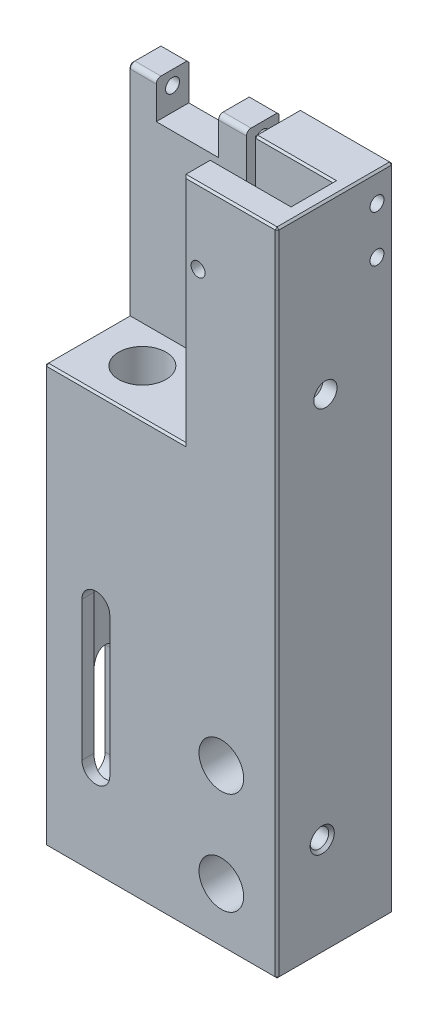
from build123d import *

# Parameters (mm, degrees)
SKETCH1_W                                         = 25
SKETCH1_H                                         = 70
BOSS_EXTRUDE1_DEPTH                               = 6.25
SKETCH2_R                                         = 4
CUT_EXTRUDE1_DEPTH                                = 35
SKETCH3_R                                         = 2.55
CUT_EXTRUDE2_DEPTH                                = 38.687033579
SKETCH5_W                                         = 9
SKETCH5_H                                         = 25
CUT_EXTRUDE3_DEPTH                                = 15
CUT_EXTRUDE4_DEPTH                                = 5
SKETCH7_R                                         = 1.75
CUT_EXTRUDE5_DEPTH                                = 6
HOLE_SIZE_PER_HEX_SOCKET_SCREW_TYPE_1_D           = 4.8
HOLE_SIZE_PER_HEX_SOCKET_SCREW_TYPE_1_CBORE_D     = 8
HOLE_SIZE_PER_HEX_SOCKET_SCREW_TYPE_1_CBORE_DEPTH = 4.6
FILLET1_R                                         = 0.5
SKETCH10_W                                        = 6.7
SKETCH10_H                                        = 5.5
SKETCH10_W_2                                      = 2.3
CUT_EXTRUDE6_DEPTH                                = 39.239377725
SKETCH11_W                                        = 2.3
SKETCH11_H                                        = 5
CUT_EXTRUDE7_DEPTH                                = 1.75
SKETCH13_W                                        = 12.7
SKETCH13_H                                        = 1.5
CUT_EXTRUDE8_DEPTH                                = 40.210967975
FILLET2_R                                         = 0.5
SKETCH14_R                                        = 0.75
CUT_EXTRUDE9_DEPTH                                = 44.463346722
SKETCH15_W                                        = 8.5
SKETCH15_H                                        = 4.5
CUT_EXTRUDE10_DEPTH                               = 25
CUT_EXTRUDE11_REACH                               = 45.463
CUT_EXTRUDE11_END_RADIUS                          = 4
SKETCH17_R                                        = 0.6
CUT_EXTRUDE12_DEPTH                               = 15
SKETCH18_R                                        = 0.75
CUT_EXTRUDE13_DEPTH                               = 40.210968006
CUT_EXTRUDE14_DEPTH                               = 7
CHAMFER1_SIZE                                     = 0.2
SKETCH20_R                                        = 1
CUT_EXTRUDE15_DEPTH                               = 19
CHAMFER2_SIZE                                     = 0.3
SKETCH21_R                                        = 1.25
CUT_EXTRUDE16_DEPTH                               = 19
CUT_EXTRUDE17_REACH                               = 45.463
SKETCH22_R                                        = 0.75
CHAMFER3_SIZE                                     = 0.2


with BuildPart() as part:
    # Sketch1 → Boss-Extrude1 (new, symmetric)
    with BuildSketch(Plane.XY):
        Rectangle(SKETCH1_W, SKETCH1_H)
    extrude(amount=BOSS_EXTRUDE1_DEPTH, both=True)

    # Sketch2 → Cut-Extrude1 (cut)
    with BuildSketch(Plane.XZ.offset(35)):
        with Locations(Location((-7, 1.25, 0), (0, 0, 270))):
            Circle(SKETCH2_R)
    extrude(amount=-CUT_EXTRUDE1_DEPTH, mode=Mode.SUBTRACT)

    # Sketch3 → Cut-Extrude2 (cut, through all)
    with BuildSketch(Plane.XZ):
        with Locations(Location((-7, 1.25, 0), (0, 0, 270))):
            Circle(SKETCH3_R)
    extrude(amount=-CUT_EXTRUDE2_DEPTH, mode=Mode.SUBTRACT)

    # Sketch5 → Cut-Extrude3 (cut)
    with BuildSketch(Plane.ZY.offset(12.5)):
        with Locations((1.75, 22.5)):
            Rectangle(SKETCH5_W, SKETCH5_H)
    extrude(amount=-CUT_EXTRUDE3_DEPTH, mode=Mode.SUBTRACT)

    # Sketch6 → Cut-Extrude4 (cut)
    with BuildSketch(Plane.XY.offset(6.25)):
        with BuildLine():
            Line((-5.5, -10), (-5.5, -25))
            ThreePointArc((-5.5, -25), (-7, -26.5), (-8.5, -25))
            Line((-8.5, -25), (-8.5, -10))
            ThreePointArc((-8.5, -10), (-7, -8.5), (-5.5, -10))
        make_face()
    extrude(amount=-CUT_EXTRUDE4_DEPTH, mode=Mode.SUBTRACT)

    # Sketch7 → Cut-Extrude5 (cut)
    with BuildSketch(Plane(origin=(0, 0, -6.25), x_dir=(-1, 0, 0), z_dir=(0, 0, -1))):
        with Locations((7, -16.07780101)):
            Circle(SKETCH7_R)
    extrude(amount=-CUT_EXTRUDE5_DEPTH, mode=Mode.SUBTRACT)

    # Hole size (per hex socket screw type) 1 (through all)
    with Locations(Plane(origin=(6.5, -29, -6.25), x_dir=(-1, 0, 0), z_dir=(0, 0, -1))):
        with Locations((0, 0), (0, 11)):
            CounterBoreHole(HOLE_SIZE_PER_HEX_SOCKET_SCREW_TYPE_1_D / 2, HOLE_SIZE_PER_HEX_SOCKET_SCREW_TYPE_1_CBORE_D / 2, HOLE_SIZE_PER_HEX_SOCKET_SCREW_TYPE_1_CBORE_DEPTH)

    # Fillet1
    fillet1_edges = [part.edges().sort_by_distance(p)[0] for p in [
        (-5, 35, -2.75),
    ]]
    fillet(fillet1_edges, radius=FILLET1_R)

    # Sketch10 → Cut-Extrude6 (cut, through all)
    with BuildSketch(Plane.XY.offset(-2.75)):
        with Locations((-6.15, 32.25)):
            Rectangle(SKETCH10_W, SKETCH10_H)
        with Locations((1.35, 32.25)):
            Rectangle(SKETCH10_W_2, SKETCH10_H)
    extrude(amount=-CUT_EXTRUDE6_DEPTH, mode=Mode.SUBTRACT)

    # Sketch11 → Cut-Extrude7 (cut)
    with BuildSketch(Plane.XY.offset(-2.75)):
        with Locations((1.35, 27)):
            Rectangle(SKETCH11_W, SKETCH11_H)
    extrude(amount=-CUT_EXTRUDE7_DEPTH, mode=Mode.SUBTRACT)

    # Sketch13 → Cut-Extrude8 (cut, through all)
    with BuildSketch(Plane(origin=(0, 0, -6.25), x_dir=(-1, 0, 0), z_dir=(0, 0, -1))):
        with Locations((6.15, 34.25)):
            Rectangle(SKETCH13_W, SKETCH13_H)
    extrude(amount=-CUT_EXTRUDE8_DEPTH, mode=Mode.SUBTRACT)

    # Fillet2
    fillet2_edges = [part.edges().sort_by_distance(p)[0] for p in [
        (-11, 33.5, -2.75),
        (-1.3, 33.5, -2.75),
    ]]
    fillet(fillet2_edges, radius=FILLET2_R)

    # Sketch14 → Cut-Extrude9 (cut, through all)
    with BuildSketch(Plane.ZY.offset(12.5)):
        with Locations(Location((-4.5, 32, 0), (0, 0, 270))):
            Circle(SKETCH14_R)
    extrude(amount=-CUT_EXTRUDE9_DEPTH, mode=Mode.SUBTRACT)

    # Sketch15 → Cut-Extrude10 (cut)
    with BuildSketch(Plane(origin=(0, 35, 0), x_dir=(1, 0, 0), z_dir=(0, 1, 0))):
        with Locations((6.75, -1)):
            Rectangle(SKETCH15_W, SKETCH15_H)
    extrude(amount=-CUT_EXTRUDE10_DEPTH, mode=Mode.SUBTRACT)

    # Cut-Extrude11: up to this cylinder (the profile starts outside it)
    cut_extrude11_end = Plane(origin=(-7, -24.5, 1.25), z_dir=(0, -1, 0)) * Cylinder(CUT_EXTRUDE11_END_RADIUS, 99.926, mode=Mode.PRIVATE)
    # Sketch16 → Cut-Extrude11 (cut, up to the surface)
    with BuildSketch(Plane.ZY.offset(12.5), mode=Mode.PRIVATE) as cut_extrude11_sk1:
        with BuildLine():
            Line((-0.25, -29.5), (-0.25, -19.5))
            ThreePointArc((-0.25, -19.5), (1.25, -18), (2.75, -19.5))
            Line((2.75, -19.5), (2.75, -29.5))
            ThreePointArc((2.75, -29.5), (1.25, -31), (-0.25, -29.5))
        make_face()
    cut_extrude11_tool1 = extrude(cut_extrude11_sk1.sketch, amount=-CUT_EXTRUDE11_REACH, mode=Mode.PRIVATE) - cut_extrude11_end
    add(cut_extrude11_tool1.solids().sort_by_distance((-12.5, -24.5, 1.25))[0], mode=Mode.SUBTRACT)

    # Sketch17 → Cut-Extrude12 (cut)
    with BuildSketch(Plane.ZY.offset(12.5)):
        with Locations(Location((-5.05, 15.2, 0), (0, 0, 270))):
            Circle(SKETCH17_R)
        with Locations(Location((-5.05, 12, 0), (0, 0, 270))):
            Circle(SKETCH17_R)
        with Locations(Location((-5.05, 7.5, 0), (0, 0, 270))):
            Circle(SKETCH17_R)
    extrude(amount=-CUT_EXTRUDE12_DEPTH, mode=Mode.SUBTRACT)

    # Sketch18 → Cut-Extrude13 (cut, through all)
    with BuildSketch(Plane.XY.offset(6.25)):
        with Locations((4, 27)):
            Circle(SKETCH18_R)
    extrude(amount=-CUT_EXTRUDE13_DEPTH, mode=Mode.SUBTRACT)

    # Sketch19 → Cut-Extrude14 (cut)
    with BuildSketch(Plane(origin=(0, 0, -6.25), x_dir=(-1, 0, 0), z_dir=(0, 0, -1))):
        with BuildLine():
            Line((-9.5, 25), (-7.5, 25))
            ThreePointArc((-7.5, 25), (-5.5, 23), (-7.5, 21))
            Line((-7.5, 21), (-9.5, 21))
            ThreePointArc((-9.5, 21), (-11.5, 23), (-9.5, 25))
        make_face()
    extrude(amount=-CUT_EXTRUDE14_DEPTH, mode=Mode.SUBTRACT)

    # Chamfer1
    chamfer1_edges = [part.edges().sort_by_distance(p)[0] for p in [
        (-5.25, -16.07780101, -6.25),
    ]]
    chamfer(chamfer1_edges, length=CHAMFER1_SIZE)

    # Sketch20 → Cut-Extrude15 (cut)
    with BuildSketch(Plane(origin=(12.5, 0, 0), x_dir=(0, 0, -1), z_dir=(1, 0, 0))):
        with Locations(Location((-1.395118476, -24.342551418, 0), (0, 0, 90))):
            Circle(SKETCH20_R)
    extrude(amount=-CUT_EXTRUDE15_DEPTH, mode=Mode.SUBTRACT)

    # Chamfer2
    chamfer2_edges = [part.edges().sort_by_distance(p)[0] for p in [
        (12.5, -25.342551418, 1.395118476),
    ]]
    chamfer(chamfer2_edges, length=CHAMFER2_SIZE)

    # Sketch21 → Cut-Extrude16 (cut)
    with BuildSketch(Plane(origin=(12.5, 0, 0), x_dir=(0, 0, -1), z_dir=(1, 0, 0))):
        with Locations(Location((-1.05, 17, 0), (0, 0, 90))):
            Circle(SKETCH21_R)
    extrude(amount=-CUT_EXTRUDE16_DEPTH, mode=Mode.SUBTRACT)

    # Cut-Extrude17: up to this face of the body (flat: up to its plane)
    cut_extrude17_end = Plane(part.part.faces().sort_by_distance((2.5, 25.799312688, -2.908885788))[0])
    # Sketch22 → Cut-Extrude17 (cut, up to the picked face)
    with BuildSketch(Plane(origin=(12.5, 0, 0), x_dir=(0, 0, -1), z_dir=(1, 0, 0)), mode=Mode.PRIVATE) as cut_extrude17_sk1:
        with Locations(Location((4.5, 26.993941921, 0), (0, 0, 90))):
            Circle(SKETCH22_R)
    cut_extrude17_tool1 = split(extrude(cut_extrude17_sk1.sketch, amount=-CUT_EXTRUDE17_REACH, mode=Mode.PRIVATE), bisect_by=cut_extrude17_end, keep=Keep.BOTH, mode=Mode.PRIVATE)
    add(cut_extrude17_tool1.solids().sort_by(Axis((12.5, 26.993942, -4.5), (-1, 0, 0)))[0], mode=Mode.SUBTRACT)

    # Chamfer3
    chamfer3_edges = [part.edges().sort_by_distance(p)[0] for p in [
        (-12.5, -0.75, -6.25),
        (-11, 33.5, -6.25),
        (-1.3, 33.5, -6.25),
        (0, -35, 6.25),
        (-12.5, 21.5, -2.75),
        (-12.5, 33.5, -4.75),
        (-12.5, 33.353553391, -2.896446609),
        (2.5, 35, -3.75),
        (6.75, 35, 3.25),
        (11, 35, 1),
        (6.75, 35, -1.25),
        (2.5, 22.5, -1.25),
        (2.5, 22.5, 3.25),
        (-12.5, -12.5, 6.25),
        (-5, 10, 6.25),
        (2.5, 22.5, 6.25),
        (-12.5, 10, 1.75),
        (12.5, 0, 6.25),
        (0, -35, -6.25),
        (7.5, 35, -6.25),
        (12.5, 0, -6.25),
        (12.5, -35, 0),
        (-12.5, -35, 0),
        (12.5, 35, 0),
        (7.5, 35, 6.25),
    ]]
    chamfer(chamfer3_edges, length=CHAMFER3_SIZE)


solid = part.part
